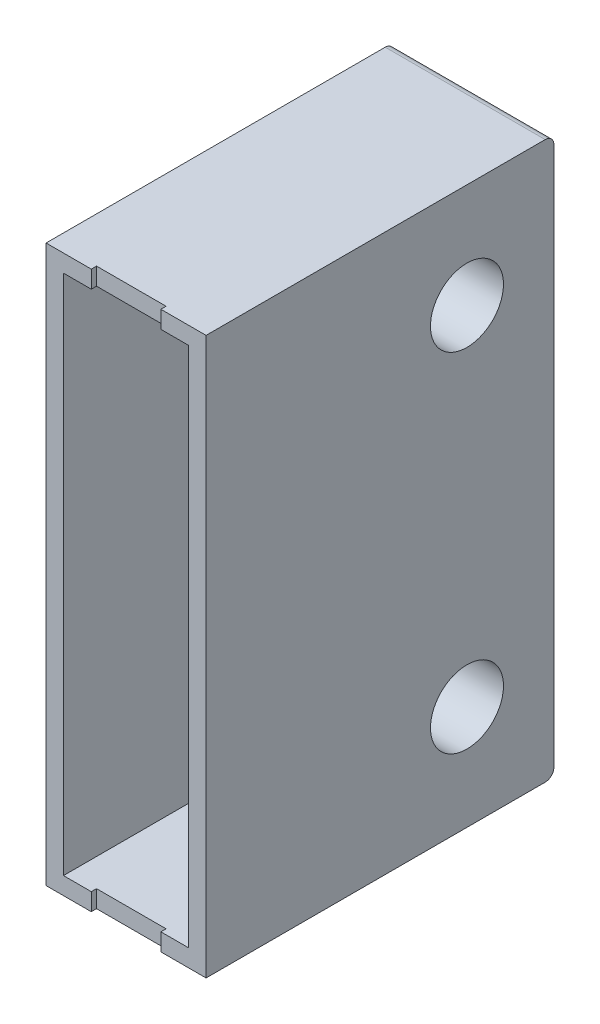
from build123d import *

# Parameters (mm, degrees)
BOSS_EXTRUDE1_DEPTH = 32
SKETCH2_R           = 2.1
CUT_EXTRUDE1_DEPTH  = 35.76550014
SKETCH3_R           = 1.740904785
BOSS_EXTRUDE2_DEPTH = 0.1
SKETCH4_R           = 3.5
BOSS_EXTRUDE3_DEPTH = 4
SKETCH5_R           = 2.5
BOSS_EXTRUDE4_DEPTH = 62
FILLET1_R           = 0.2
FILLET2_R           = 0.5
SKETCH6_W           = 7.2
SKETCH6_H           = 30
CUT_EXTRUDE2_DEPTH  = 19
SKETCH7_W           = 16.27166032
SKETCH7_H           = 23.629900988
CUT_EXTRUDE3_DEPTH  = 74.5
SKETCH8_R           = 1.9
CUT_EXTRUDE4_DEPTH  = 17.5
SKETCH9_R           = 3.1
SKETCH9_R_2         = 2.1
BOSS_EXTRUDE5_DEPTH = 7.2


with BuildPart() as part:
    # Sketch1 → Boss-Extrude1 (new body)
    with BuildSketch(Plane(origin=(0, 0, 0), x_dir=(1, 0, 0), z_dir=(0, 1, 0))):
        Polygon((2, -10), (4.6, -10), (4.6, 10), (-4.6, 10), (-4.6, -10), (-2, -10), (-2, -9.7), (2, -9.7), align=None)
    extrude(amount=BOSS_EXTRUDE1_DEPTH)

    # Sketch2 → Cut-Extrude1 (cut, through all)
    with BuildSketch(Plane(origin=(4.6, 0, 0), x_dir=(0, 0, -1), z_dir=(1, 0, 0))):
        with Locations((5, 26)):
            Circle(SKETCH2_R)
        with Locations((5, 6)):
            Circle(SKETCH2_R)
    extrude(amount=-CUT_EXTRUDE1_DEPTH, mode=Mode.SUBTRACT)

    # Sketch3 → Boss-Extrude2 (add)
    with BuildSketch(Plane(origin=(0, 0, -10), x_dir=(-1, 0, 0), z_dir=(0, 0, -1))):
        with Locations((0, 18.961857961)):
            Circle(SKETCH3_R)
    extrude(amount=BOSS_EXTRUDE2_DEPTH)

    # Sketch4 → Boss-Extrude3 (add)
    with BuildSketch(Plane.XZ):
        with Locations(Location((0, 0, 0), (0, 0, 270))):
            Circle(SKETCH4_R)
    extrude(amount=BOSS_EXTRUDE3_DEPTH)

    # Sketch5 → Boss-Extrude4 (add)
    with BuildSketch(Plane.XZ.offset(4)):
        with Locations(Location((0, 0, 0), (0, 0, 270))):
            Circle(SKETCH5_R)
    extrude(amount=BOSS_EXTRUDE4_DEPTH)

    # Fillet1
    fillet1_edges = [part.edges().sort_by_distance(p)[0] for p in [
        (0, -4, 3.5),
    ]]
    fillet(fillet1_edges, radius=FILLET1_R)

    # Fillet2
    fillet2_edges = [part.edges().sort_by_distance(p)[0] for p in [
        (0, 0, -10),
        (0, 32, -10),
    ]]
    fillet(fillet2_edges, radius=FILLET2_R)

    # Sketch6 → Cut-Extrude2 (cut)
    with BuildSketch(Plane.XY.offset(10)):
        with Locations((0, 16)):
            Rectangle(SKETCH6_W, SKETCH6_H)
    extrude(amount=-CUT_EXTRUDE2_DEPTH, mode=Mode.SUBTRACT)

    # Sketch7 → Cut-Extrude3 (cut)
    with BuildSketch(Plane.XZ):
        with Locations((-4.097079532, -5.79987022)):
            Rectangle(SKETCH7_W, SKETCH7_H)
    extrude(amount=CUT_EXTRUDE3_DEPTH, mode=Mode.SUBTRACT)

    # Sketch8 → Cut-Extrude4 (cut)
    with BuildSketch(Plane.XZ):
        with Locations(Location((0, 0, 0), (0, 0, 270))):
            Circle(SKETCH8_R)
    extrude(amount=-CUT_EXTRUDE4_DEPTH, mode=Mode.SUBTRACT)

    # Sketch9 → Boss-Extrude5 (add)
    # profile 1 of 2: a face of its own
    with BuildSketch(Plane.ZY.offset(-3.6)):
        with Locations(Location((-5, 26, 0), (0, 0, 90))):
            Circle(SKETCH9_R)
        with Locations(Location((-5, 26, 0), (0, 0, 180))):
            Circle(SKETCH9_R_2, mode=Mode.SUBTRACT)
    # profile 2 of 2: a face of its own
    with BuildSketch(Plane.ZY.offset(-3.6)):
        with Locations(Location((-5, 6, 0), (0, 0, 90))):
            Circle(SKETCH9_R)
        with Locations(Location((-5, 6, 0), (0, 0, 180))):
            Circle(SKETCH9_R_2, mode=Mode.SUBTRACT)
    extrude(amount=BOSS_EXTRUDE5_DEPTH)


solid = part.part
